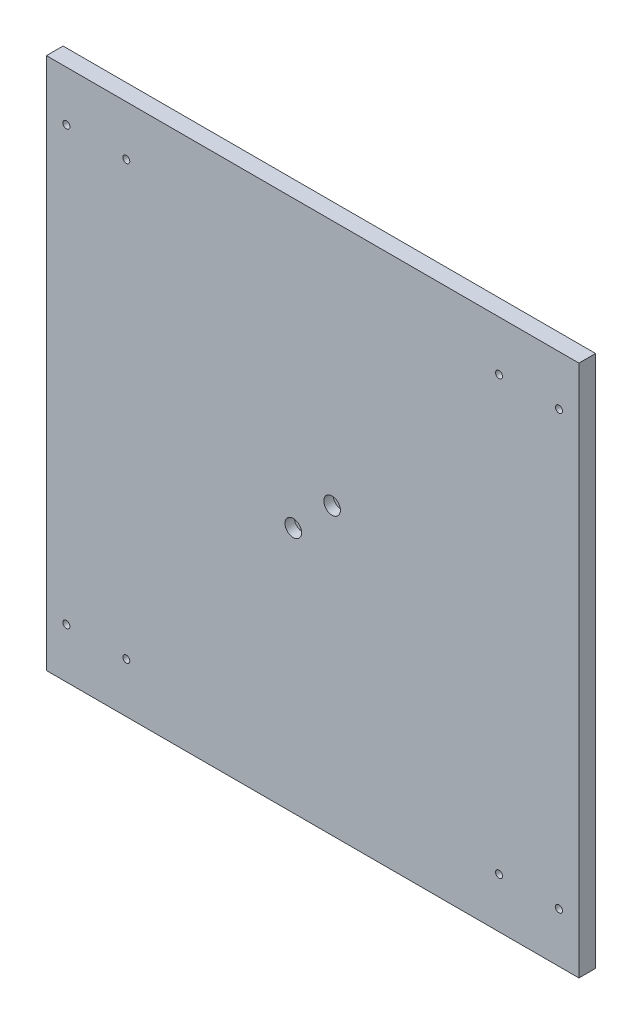
SolidWorks part; units mm, degrees
material "6061 合金"
ref_plane "前视基准面" through (0, 0, 0) normal (0, 0, 1) x (1, 0, 0)
ref_plane "上视基准面" through (0, 0, 0) normal (0, 1, 0) x (1, 0, 0)
ref_plane "右视基准面" through (0, 0, 0) normal (1, 0, 0) x (0, 0, -1)
sketch "草图1" plane through (0, 0, 0) normal (0, 0, 1) x (1, 0, 0)
  line L1 (-160, 160) -> (160, 160)
  line L2 (-160, 160) -> (-160, -160)
  line L3 (-160, -160) -> (160, -160)
  line L4 (160, 160) -> (160, -160)
  line L5 (-160, 160) -> (160, -160) construction
  line L6 (-160, -160) -> (160, 160) construction
  point P0 (0, 0)
  dimension "D1" = 320
  dimension "D2" = 320
extrude "凸台-拉伸1" add sketch "草图1" along normal blind 10
hole_wizard "打孔尺寸(%根据)内六角圆柱头螺钉的类型1" positions "草图3" profile "草图2" counterbore size "M5" standard "GB"
sketch "草图3" plane through (0, 0, 10) normal (0, 0, 1) x (1, 0, 0)
  line L0 (-173.7046, 0) -> (210.9299, 0) construction
  line L2 (0, 84.914) -> (0, -124.593) construction
  line L3 (-35.6289, -35.6289) -> (35.6289, 35.6289) construction
  line L4 (0, 0) -> (-31.3991, 31.3991) construction
  point P0 (-11.6673, -11.6673)
  point P2 (11.6673, 11.6673)
  dimension "D1" = 33
  dimension "D4" = 45
sketch "草图2" plane through (-11.6673, -11.6673, 10) normal (1, 0, 0) x (0, -1, 0)
  line L0 (0, 0) -> (0, 11.6524)
  line L1 (0, 11.6524) -> (2.75, 10)
  line L2 (2.75, 10) -> (2.75, 5.7)
  line L3 (2.75, 5.7) -> (5, 5.7)
  line L4 (5, 5.7) -> (5, 0)
  line L5 (5, 0) -> (0, 0)
  line L10 (0, 11.6524) -> (-2.75, 10) construction
  line L11 (0, -6.35) -> (0, 107.95) construction
  dimension "孔直径" = 5.5
  dimension "孔深度" = 10
  dimension "柱形沉头孔直径" = 10
  dimension "柱形沉头孔深度" = 5.7
  dimension "导头角度" = 118
hole_wizard "M5 螺纹孔1" positions "草图5" profile "草图6" tap size "M5" standard "GB" end condition through all
sketch "草图5" plane through (0, 0, 0) normal (0, 0, -1) x (-1, 0, 0)
  line L0 (0, 0) -> (-160, 160) construction
  line L2 (-148, 130) -> (-112, 130) construction
  line L4 (-160, -160) -> (-160, 160) construction
  line L5 (-160, 160) -> (160, 160) construction
  point P0 (-148, 130)
  point P2 (-112, 130)
  dimension "D1" = 36
  dimension "D2" = 12
  dimension "D3" = 30
sketch "草图6" plane through (148, 130, 0) normal (1, 0, 0) x (0, 1, 0)
  line L0 (0, 0) -> (0, 10)
  line L1 (0, 10) -> (2.1, 10)
  line L2 (2.1, 10) -> (2.1, 0)
  line L5 (2.1, 0) -> (0, 0)
  line L11 (0, -6.35) -> (0, 107.95) construction
  dimension "通孔螺纹孔钻头直径" = 4.2
  dimension "通孔螺纹孔钻头深度" = 10
cosmetic thread "孔螺蚊线1" parameters "D2"=5
cosmetic thread "孔螺蚊线2" parameters "D2"=5
mirror "镜向1" about plane through (0, 0, 0) normal (0, 1, 0) of "M5 螺纹孔1"
mirror "镜向2" about plane through (0, 0, 0) normal (1, 0, 0) of "镜向1", "M5 螺纹孔1"
